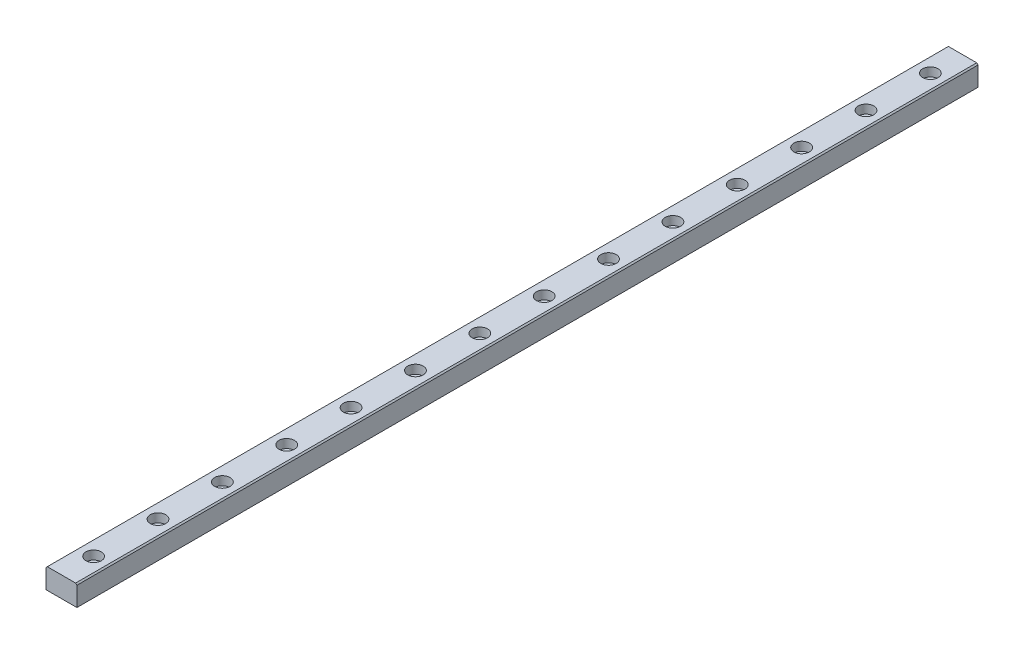
SolidWorks part; units mm, degrees
ref_plane "前视基准面" through (0, 0, 0) normal (0, 0, 1) x (1, 0, 0)
ref_plane "上视基准面" through (0, 0, 0) normal (0, 1, 0) x (1, 0, 0)
ref_plane "右视基准面" through (0, 0, 0) normal (1, 0, 0) x (0, 0, -1)
sketch "草图1" plane through (0, 0, 0) normal (0, 0, 1) x (1, 0, 0)
  line L1 (6, 4) -> (-6, 4)
  line L2 (6, 4) -> (6, -4)
  line L3 (6, -4) -> (-6, -4)
  line L4 (-6, 4) -> (-6, -4)
  line L5 (6, 4) -> (-6, -4) construction
  line L6 (6, -4) -> (-6, 4) construction
  point P0 (0, 0)
  dimension "D1" = 12
  dimension "D2" = 8
extrude "凸台-拉伸1" add sketch "草图1" along normal blind 350
chamfer "倒角1" distance 0.5 distance2 0.5 1 edges at (6, 4, 175)
chamfer "倒角2" distance 0.5 distance2 0.5 1 edges at (-6, 4, 175)
hole_wizard "打孔尺寸根据内六角圆柱头螺钉的类型1" positions "草图3" profile "草图2" counterbore size "M3" standard "Gb" end condition through all
sketch "草图3" plane through (0, 4, 0) normal (0, 1, 0) x (1, 0, 0)
  line L0 (5.5, 0) -> (-5.5, 0) construction
  point P0 (0, -12.5)
  dimension "D1" = 12.5
sketch "草图2" plane through (0, 4, 12.5) normal (1, 0, 0) x (0, 0, 1)
  line L0 (0, 0) -> (0, 8)
  line L1 (0, 8) -> (1.7, 8)
  line L3 (1.7, 8) -> (1.7, 3.4)
  line L4 (1.7, 3.4) -> (3, 3.4)
  line L5 (3, 3.4) -> (3, 0)
  line L7 (3, 0) -> (0, 0)
  line L11 (0, -6.35) -> (0, 107.95) construction
  dimension "通孔孔直径" = 3.4
  dimension "通孔孔深度" = 8
  dimension "柱形沉头孔直径" = 6
  dimension "柱形沉头孔深度" = 3.4
pattern_linear "阵列(线性)1" count 14 spacing 25 along (0, 0, 1) of "打孔尺寸根据内六角圆柱头螺钉的类型1"
